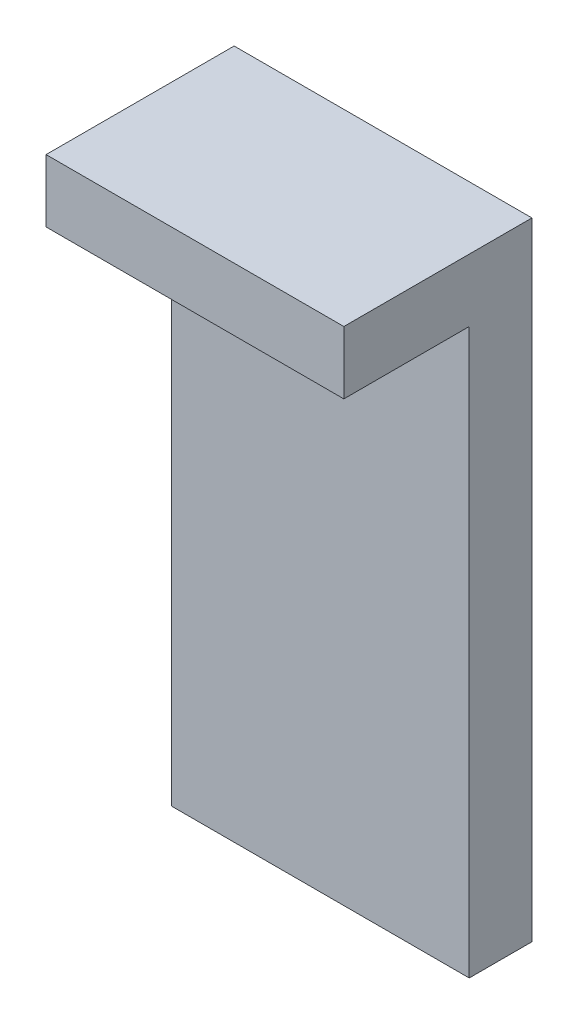
SolidWorks part; units mm, degrees
ref_plane "前视基准面" through (0, 0, 0) normal (0, 0, 1) x (1, 0, 0)
ref_plane "上视基准面" through (0, 0, 0) normal (0, 1, 0) x (1, 0, 0)
ref_plane "右视基准面" through (0, 0, 0) normal (1, 0, 0) x (0, 0, -1)
sketch "草图1" plane through (0, 0, 0) normal (0, 0, 1) x (1, 0, 0)
  line L1 (-19, -40) -> (19, -40)
  line L2 (-19, -40) -> (-19, 40)
  line L3 (-19, 40) -> (19, 40)
  line L4 (19, -40) -> (19, 40)
  line L5 (-19, -40) -> (19, 40) construction
  line L6 (-19, 40) -> (19, -40) construction
  point P0 (0, 0)
  dimension "D1" = 38
  dimension "D2" = 80
extrude "凸台-拉伸1" add sketch "草图1" along normal mid plane 8
sketch "草图2" plane through (0, 0, 4) normal (0, 0, 1) x (1, 0, 0)
  line L0 (19, -40) -> (19, 40) construction
  line L1 (-19, 40) -> (19, 40)
  line L2 (-19, 40) -> (-19, 32)
  line L3 (-19, 32) -> (19, 32)
  line L4 (19, 40) -> (19, 32)
  dimension "D1" = 8
extrude "凸台-拉伸2" add sketch "草图2" along normal blind 16
